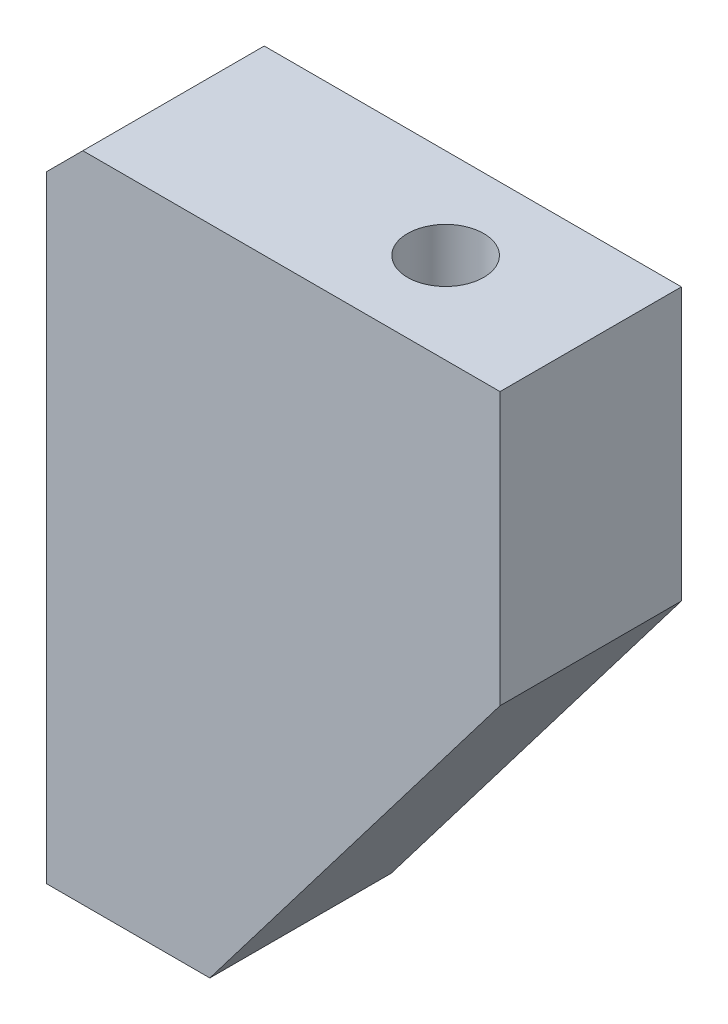
SolidWorks part; units mm, degrees
ref_plane "前视基准面" through (0, 0, 0) normal (0, 0, 1) x (1, 0, 0)
ref_plane "上视基准面" through (0, 0, 0) normal (0, 1, 0) x (1, 0, 0)
ref_plane "右视基准面" through (0, 0, 0) normal (1, 0, 0) x (0, 0, -1)
sketch "草图1" plane through (0, 0, 0) normal (0, 0, 1) x (1, 0, 0)
  line L0 (-64.6341, -10.7968) -> (-39.6341, -10.7968)
  line L2 (-39.6341, -25.7968) -> (-55.6341, -46.7968)
  line L3 (-55.6341, -46.7968) -> (-64.6341, -46.7968)
  line L4 (-64.6341, -10.7968) -> (-64.6341, -46.7968)
  line L5 (-39.6341, -10.7968) -> (-39.6341, -25.7968)
  dimension "D1" = 25
  dimension "D2" = 36
  dimension "D3" = 9
  dimension "D4" = 15
extrude "凸台-拉伸1" add sketch "草图1" along normal blind 10
hole_wizard "M5 螺纹孔2" positions "草图3" profile "草图2" tap size "M5" standard "Iso"
sketch "草图3" plane through (0, -10.7968, 0) normal (0, 1, 0) x (1, 0, 0)
  line L1 (-39.6341, -10) -> (-39.6341, 0) construction
  line L3 (-39.6341, 0) -> (-64.6341, 0) construction
  point P0 (-47.6341, -5)
  dimension "D1" = 8
  dimension "D2" = 5
sketch "草图2" plane through (-47.6341, -10.7968, 5) normal (1, 0, 0) x (0, 0, 1)
  line L0 (0, 0) -> (0, 14.2618)
  line L1 (0, 14.2618) -> (2.1, 13)
  line L2 (2.1, 13) -> (2.1, 0)
  line L5 (2.1, 0) -> (0, 0)
  line L10 (0, 14.2618) -> (-2.1, 13) construction
  line L11 (0, -6.35) -> (0, 107.95) construction
  dimension "螺纹孔钻头直径" = 4.2
  dimension "螺纹孔钻头深度" = 13
  dimension "导头角度" = 118
cosmetic thread "孔螺蚊线1" parameters "D1"=10, "D2"=5
hole_wizard "M5 螺纹孔1" positions "草图5" profile "草图4" tap size "M5" standard "Iso"
sketch "草图5" plane through (-64.6341, 0, 0) normal (-1, 0, 0) x (0, 0, 1)
  line L0 (10, -10.7968) -> (0, -10.7968) construction
  line L1 (10, -10.7968) -> (10, -46.7968) construction
  point P0 (5, -18.7968)
  point P2 (5, -38.7968)
  dimension "D1" = 8
  dimension "D2" = 20
  dimension "D3" = 5
sketch "草图4" plane through (-64.6341, -18.7968, 5) normal (0, 1, 0) x (0, 0, 1)
  line L0 (0, 0) -> (0, 14.2618)
  line L1 (0, 14.2618) -> (2.1, 13)
  line L2 (2.1, 13) -> (2.1, 0)
  line L5 (2.1, 0) -> (0, 0)
  line L10 (0, 14.2618) -> (-2.1, 13) construction
  line L11 (0, -6.35) -> (0, 107.95) construction
  dimension "螺纹孔钻头直径" = 4.2
  dimension "螺纹孔钻头深度" = 13
  dimension "导头角度" = 118
cosmetic thread "孔螺蚊线2" parameters "D1"=10, "D2"=5
cosmetic thread "孔螺蚊线3" parameters "D1"=10, "D2"=5
chamfer "倒角1" distance 2 angle 45 1 edges at (-64.6341, -10.7968, 5)
